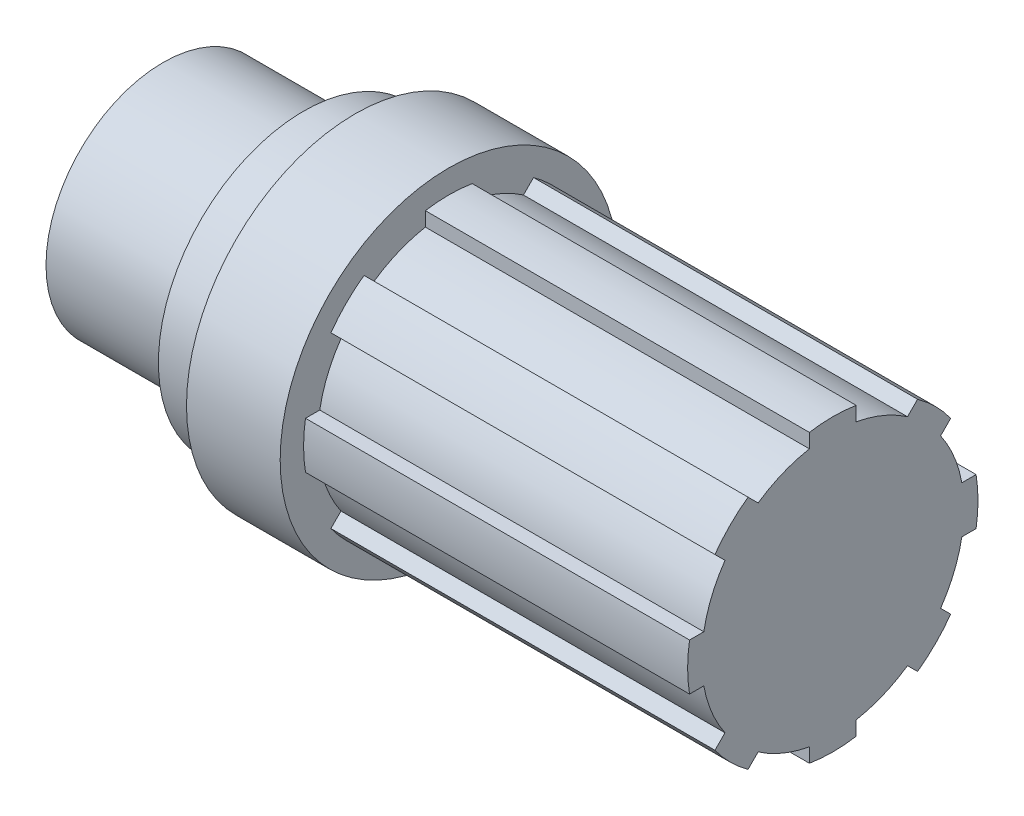
from build123d import *

# Parameters (mm, degrees)
BOSS_EXTRUDE1_DEPTH = 82
CIRPATTERN1_COUNT   = 8
SKETCH3_R           = 25
BOSS_EXTRUDE2_DEPTH = 30


with BuildPart() as part:
    # Sketch1 → Revolve1 (revolve)
    with BuildSketch(Plane(origin=(0, 0, 0), x_dir=(1, 0, 0), z_dir=(0, 1, 0))):
        Polygon((0, 0), (0, 31), (11, 31), (11, 36), (31, 36), (31, 28), (113, 28), (113, 0), align=None)
    revolve(axis=Axis((113, 0, 0), (-1, 0, 0)))

    # Sketch2 → Boss-Extrude1 (add)
    with BuildSketch(Plane(origin=(113, 0, 0), x_dir=(0, 0, -1), z_dir=(1, 0, 0))):
        with BuildLine():
            Line((-5, 30.594117082), (-5, 27.549954628))
            ThreePointArc((-5, 27.549954628), (0, 28), (5, 27.549954628))
            Line((5, 27.549954628), (5, 30.594117082))
            ThreePointArc((5, 30.594117082), (0, 31), (-5, 30.594117082))
        make_face()
    boss_extrude1 = extrude(amount=-BOSS_EXTRUDE1_DEPTH)

    # CirPattern1: Boss-Extrude1 ×8 about axis
    cirpattern1_axis = Axis((0, 0, 0), (1, 0, 0))
    for i in range(1, CIRPATTERN1_COUNT):
        add(boss_extrude1.rotate(cirpattern1_axis, i * 360 / CIRPATTERN1_COUNT))

    # Sketch3 → Boss-Extrude2 (add)
    with BuildSketch(Plane.ZY):
        Circle(SKETCH3_R)
    extrude(amount=BOSS_EXTRUDE2_DEPTH)


solid = part.part
